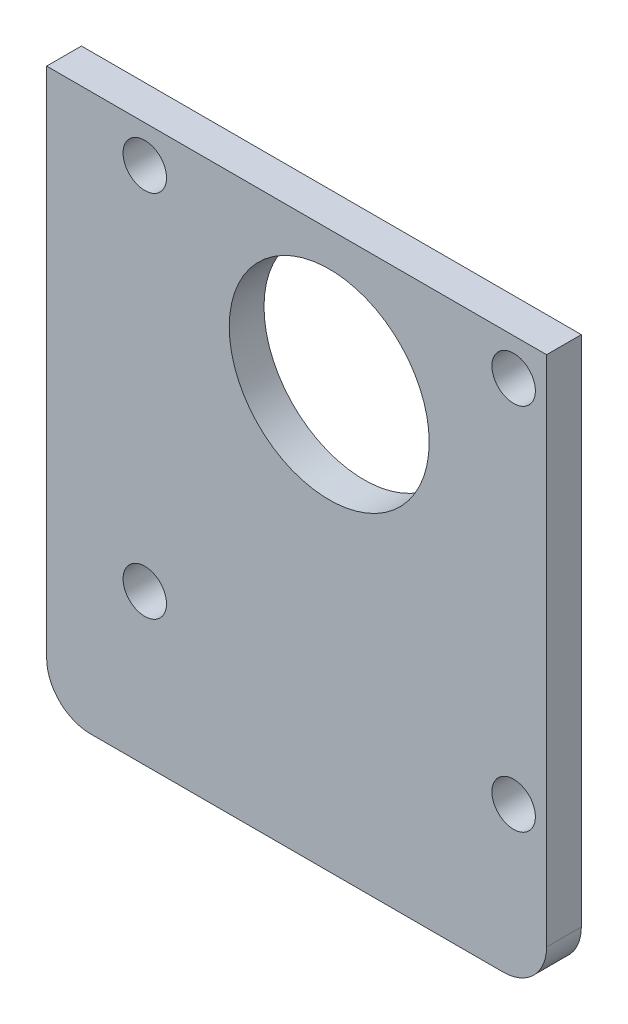
from build123d import *

# Parameters (mm, degrees)
SKETCH1_W           = 115
SKETCH1_H           = 128
BOSS_EXTRUDE1_DEPTH = 4
F_10_HOLE1_D        = 10
FILLET1_R           = 10
CUT_EXTRUDE1_REACH  = 88.407
SKETCH4_R           = 23


with BuildPart() as part:
    # Sketch1 → Boss-Extrude1 (new, symmetric)
    with BuildSketch(Plane.XY):
        Rectangle(SKETCH1_W, SKETCH1_H)
    extrude(amount=BOSS_EXTRUDE1_DEPTH, both=True)

    # Ø10 Hole1 (through all)
    with Locations(Plane.XY.offset(4)):
        with Locations((-34.926406871, 55.5), (49.926406871, 55.5), (49.926406871, -29.352813742), (-34.926406871, -29.352813742)):
            Hole(F_10_HOLE1_D / 2)

    # Fillet1
    fillet1_edges = [part.edges().sort_by_distance(p)[0] for p in [
        (57.5, -64, 0),
        (-57.5, -64, 0),
    ]]
    fillet(fillet1_edges, radius=FILLET1_R)

    # Sketch4 → Cut-Extrude1 (cut, up to next)
    with BuildSketch(Plane.XY.offset(4), mode=Mode.PRIVATE) as cut_extrude1_sk1:
        with Locations((7.5, 33.073593129)):
            Circle(SKETCH4_R)
    cut_extrude1_tool1 = extrude(cut_extrude1_sk1.sketch, amount=-CUT_EXTRUDE1_REACH, mode=Mode.PRIVATE) & part.part
    add(cut_extrude1_tool1.solids().sort_by_distance((7.5, 33.073593, 4))[0], mode=Mode.SUBTRACT)


solid = part.part
